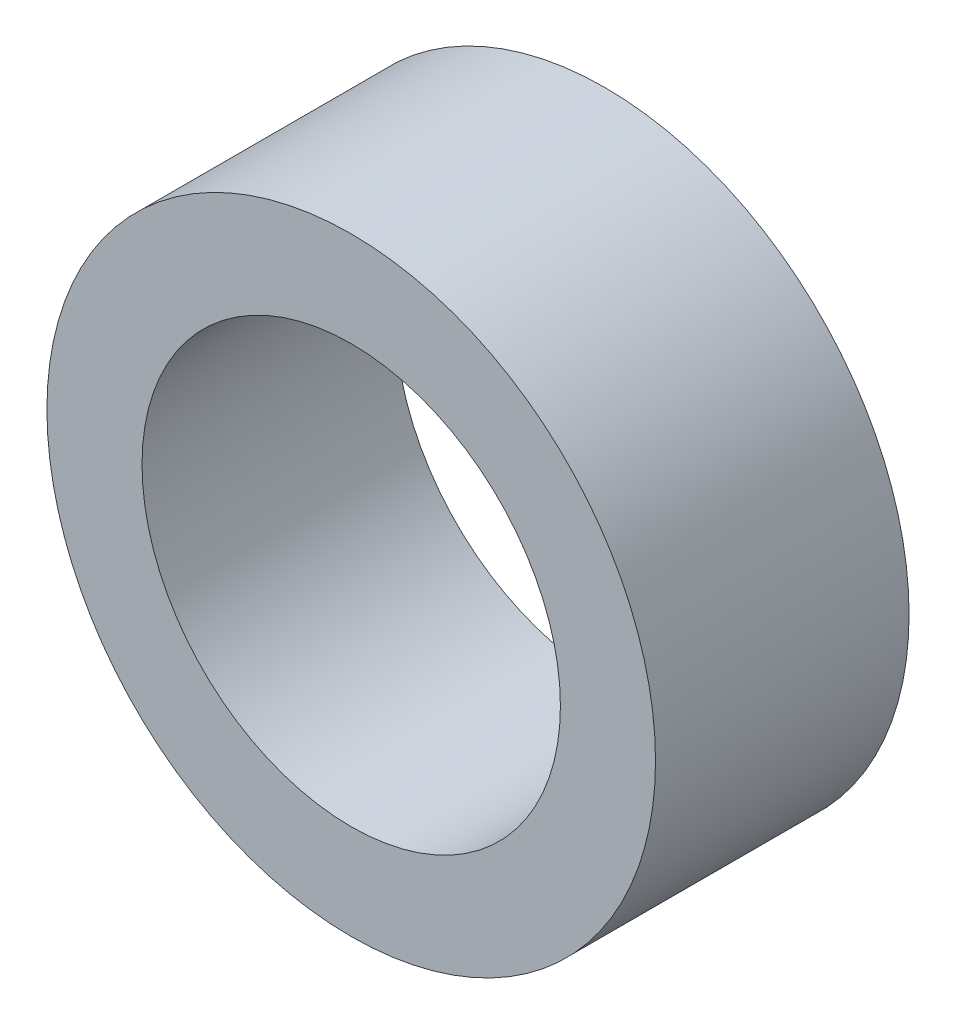
SolidWorks part; units mm, degrees
ref_plane "前视基准面" through (0, 0, 0) normal (0, 0, 1) x (1, 0, 0)
ref_plane "上视基准面" through (0, 0, 0) normal (0, 1, 0) x (1, 0, 0)
ref_plane "右视基准面" through (0, 0, 0) normal (1, 0, 0) x (0, 0, -1)
sketch "草图1" plane through (0, 0, 0) normal (0, 0, 1) x (1, 0, 0)
  circle A0 centre (0, 0) radius 8.25
  circle A1 centre (0, 0) radius 12
  dimension "D1" = 16.5
  dimension "D2" = 24
extrude "凸台-拉伸1" add sketch "草图1" along normal blind 10
